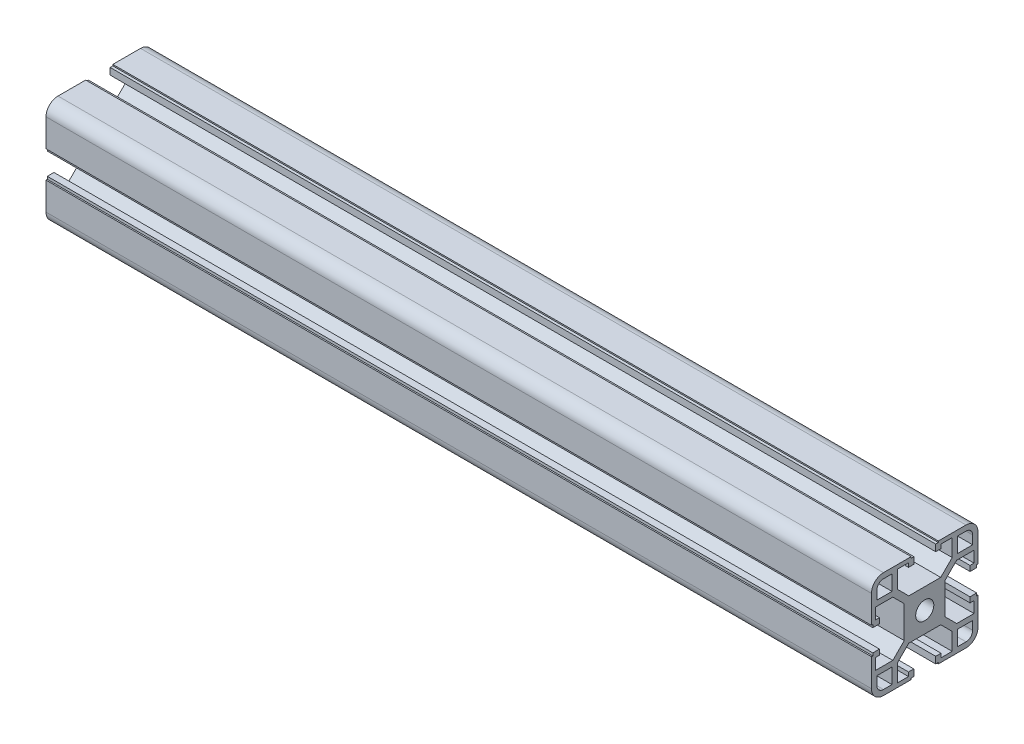
from build123d import *

# Parameters (mm, degrees)
SKETCH1_R                                 = 3.4
ALUMINIUM_PROFILE_40_X_40B_X_R4_5_1_DEPTH = 310


with BuildPart() as part:
    # Sketch1 → Aluminium profile 40 X 40B X R4.5(1) (new body)
    with BuildSketch(Plane.YZ.offset(-984.974958264)):
        with BuildLine():
            Line((-5.1, 20), (-5.1, 19.5))
            Line((-5.1, 19.5), (-4.1, 19.5))
            Line((-4.1, 19.5), (-4.1, 17))
            Line((-4.1, 17), (-6.1, 17))
            Line((-6.1, 17), (-6.1, 18.5))
            Line((-6.1, 18.5), (-10.3, 18.5))
            Line((-10.3, 18.5), (-10.3, 12))
            Line((-10.3, 12), (-6, 7.7))
            Line((-6, 7.7), (6, 7.7))
            Line((6, 7.7), (10.3, 12))
            Line((10.3, 12), (10.3, 18.5))
            Line((10.3, 18.5), (6.1, 18.5))
            Line((6.1, 18.5), (6.1, 17))
            Line((6.1, 17), (4.1, 17))
            Line((4.1, 17), (4.1, 19.5))
            Line((4.1, 19.5), (5.1, 19.5))
            Line((5.1, 19.5), (5.1, 20))
            Line((5.1, 20), (15.5, 20))
            ThreePointArc((15.5, 20), (18.681980515, 18.681980515), (20, 15.5))
            Line((20, 15.5), (20, 5.1))
            Line((20, 5.1), (19.5, 5.1))
            Line((19.5, 5.1), (19.5, 4.1))
            Line((19.5, 4.1), (17, 4.1))
            Line((17, 4.1), (17, 6.1))
            Line((17, 6.1), (18.5, 6.1))
            Line((18.5, 6.1), (18.5, 10.3))
            Line((18.5, 10.3), (12, 10.3))
            Line((12, 10.3), (7.7, 6))
            Line((7.7, 6), (7.7, -6))
            Line((7.7, -6), (12, -10.3))
            Line((12, -10.3), (18.5, -10.3))
            Line((18.5, -10.3), (18.5, -6.1))
            Line((18.5, -6.1), (17, -6.1))
            Line((17, -6.1), (17, -4.1))
            Line((17, -4.1), (19.5, -4.1))
            Line((19.5, -4.1), (19.5, -5.1))
            Line((19.5, -5.1), (20, -5.1))
            Line((20, -5.1), (20, -15.5))
            ThreePointArc((20, -15.5), (18.681980515, -18.681980515), (15.5, -20))
            Line((15.5, -20), (5.1, -20))
            Line((5.1, -20), (5.1, -19.5))
            Line((5.1, -19.5), (4.1, -19.5))
            Line((4.1, -19.5), (4.1, -17))
            Line((4.1, -17), (6.1, -17))
            Line((6.1, -17), (6.1, -18.5))
            Line((6.1, -18.5), (10.3, -18.5))
            Line((10.3, -18.5), (10.3, -12))
            Line((10.3, -12), (6, -7.7))
            Line((6, -7.7), (-6, -7.7))
            Line((-6, -7.7), (-10.3, -12))
            Line((-10.3, -12), (-10.3, -18.5))
            Line((-10.3, -18.5), (-6.1, -18.5))
            Line((-6.1, -18.5), (-6.1, -17))
            Line((-6.1, -17), (-4.1, -17))
            Line((-4.1, -17), (-4.1, -19.5))
            Line((-4.1, -19.5), (-5.1, -19.5))
            Line((-5.1, -19.5), (-5.1, -20))
            Line((-5.1, -20), (-15.5, -20))
            ThreePointArc((-15.5, -20), (-18.681980515, -18.681980515), (-20, -15.5))
            Line((-20, -15.5), (-20, -5.1))
            Line((-20, -5.1), (-19.5, -5.1))
            Line((-19.5, -5.1), (-19.5, -4.1))
            Line((-19.5, -4.1), (-17, -4.1))
            Line((-17, -4.1), (-17, -6.1))
            Line((-17, -6.1), (-18.5, -6.1))
            Line((-18.5, -6.1), (-18.5, -10.3))
            Line((-18.5, -10.3), (-12, -10.3))
            Line((-12, -10.3), (-7.7, -6))
            Line((-7.7, -6), (-7.7, 6))
            Line((-7.7, 6), (-12, 10.3))
            Line((-12, 10.3), (-18.5, 10.3))
            Line((-18.5, 10.3), (-18.5, 6.1))
            Line((-18.5, 6.1), (-17, 6.1))
            Line((-17, 6.1), (-17, 4.1))
            Line((-17, 4.1), (-19.5, 4.1))
            Line((-19.5, 4.1), (-19.5, 5.1))
            Line((-19.5, 5.1), (-20, 5.1))
            Line((-20, 5.1), (-20, 15.5))
            ThreePointArc((-20, 15.5), (-18.681980515, 18.681980515), (-15.5, 20))
            Line((-15.5, 20), (-5.1, 20))
        make_face()
        Circle(SKETCH1_R, mode=Mode.SUBTRACT)
        with BuildLine():
            Line((12.3, 18), (15.5, 18))
            ThreePointArc((15.5, 18), (17.267766953, 17.267766953), (18, 15.5))
            Line((18, 15.5), (18, 12.3))
            Line((18, 12.3), (12.3, 12.3))
            Line((12.3, 12.3), (12.3, 18))
        make_face(mode=Mode.SUBTRACT)
        with BuildLine():
            Line((-15.5, 18), (-12.3, 18))
            Line((-12.3, 18), (-12.3, 12.3))
            Line((-12.3, 12.3), (-18, 12.3))
            Line((-18, 12.3), (-18, 15.5))
            ThreePointArc((-18, 15.5), (-17.267766953, 17.267766953), (-15.5, 18))
        make_face(mode=Mode.SUBTRACT)
        with BuildLine():
            Line((-18, -12.3), (-12.3, -12.3))
            Line((-12.3, -12.3), (-12.3, -18))
            Line((-12.3, -18), (-15.5, -18))
            ThreePointArc((-15.5, -18), (-17.267766953, -17.267766953), (-18, -15.5))
            Line((-18, -15.5), (-18, -12.3))
        make_face(mode=Mode.SUBTRACT)
        with BuildLine():
            Line((12.3, -12.3), (18, -12.3))
            Line((18, -12.3), (18, -15.5))
            ThreePointArc((18, -15.5), (17.267766953, -17.267766953), (15.5, -18))
            Line((15.5, -18), (12.3, -18))
            Line((12.3, -18), (12.3, -12.3))
        make_face(mode=Mode.SUBTRACT)
    extrude(amount=ALUMINIUM_PROFILE_40_X_40B_X_R4_5_1_DEPTH)


solid = part.part
